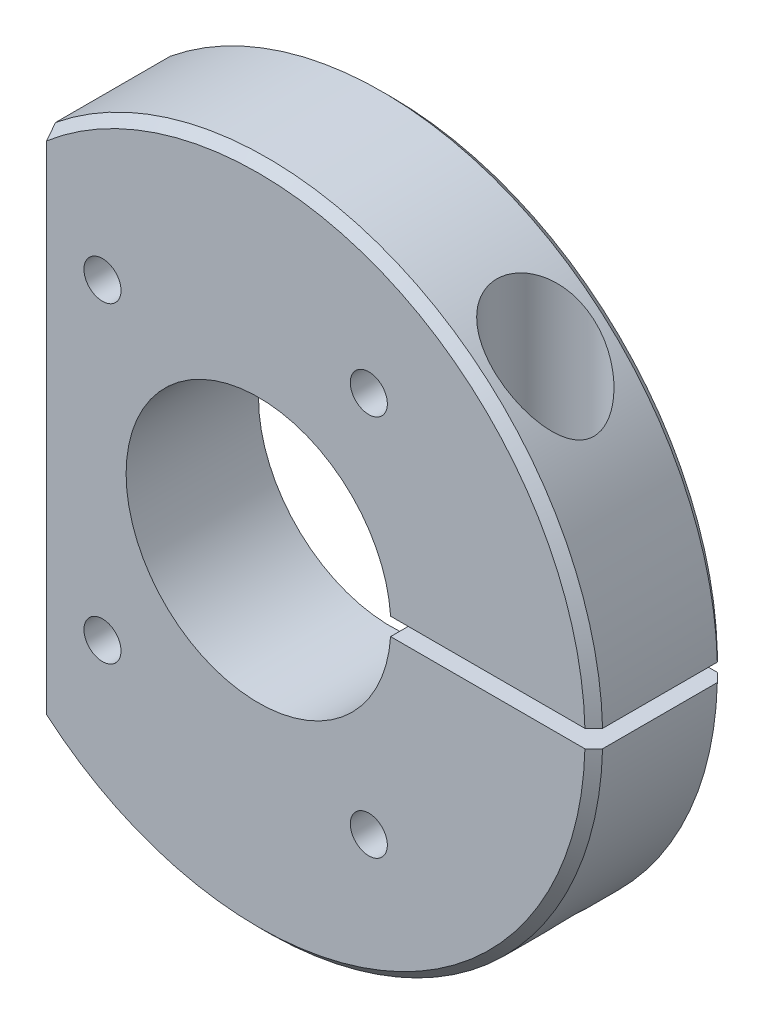
from build123d import *

# Parameters (mm, degrees)
EXTRUDE_1_DEPTH              = 15
CUT_EXTRUDE_1_DEPTH          = 56.794264938
SKETCH_3_W                   = 15
SKETCH_3_H                   = 15
HOLE_WIZARD_4_2_4_2_1_D      = 4.2
SKETCH_6_W                   = 2.5
SKETCH_6_H                   = 37
HOLE_WIZARD_M6_1_D           = 6.5
HOLE_WIZARD_M6_1_DEPTH       = 70.615180295
HOLE_WIZARD_M6_1_CBORE_D     = 11
HOLE_WIZARD_M6_1_CBORE_DEPTH = 24.615180295
CHAMFER_1_SIZE               = 1


with BuildPart() as part:
    # 草图1 → 凸台-拉伸1 (new body)
    with BuildSketch(Plane(origin=(0, 0, -7.5), x_dir=(-1, 0, 0), z_dir=(0, 0, -1))):
        with BuildLine():
            Line((24, -29.461839725), (24, 29.461839725))
            ThreePointArc((24, 29.461839725), (-38, 0), (24, -29.461839725))
        make_face()
    extrude(amount=-EXTRUDE_1_DEPTH)

    # 草图2 → 切除-拉伸1 (cut, through all)
    with BuildSketch(Plane.XY.offset(7.5)):
        with BuildLine():
            Line((37.986839826, 1), (14.966629547, 1))
            ThreePointArc((14.966629547, 1), (15, 0), (14.966629547, -1))
            Line((14.966629547, -1), (37.986839826, -1))
            ThreePointArc((37.986839826, -1), (38, 0), (37.986839826, 1))
        make_face()
    extrude(amount=-CUT_EXTRUDE_1_DEPTH, mode=Mode.SUBTRACT)

    # 草图3 → 切除-旋转1 (revolve, cut)
    with BuildSketch(Plane.XZ):
        with Locations((7.5, 0)):
            Rectangle(SKETCH_3_W, SKETCH_3_H)
    revolve(axis=Axis((0, 0, 7.5), (0, 0, -1)), mode=Mode.SUBTRACT)

    # Ø4.2 (4.2) 直径孔1 (through all)
    with Locations(Plane.XY.offset(7.5)):
        with Locations((-17.67766953, -17.67766953), (-17.67766953, 17.67766953), (12.5, 21.650635095), (12.5, -21.650635095)):
            Hole(HOLE_WIZARD_4_2_4_2_1_D / 2)

    # 草图6 → Ø5.0 (5) 直径孔1 (revolve, cut)
    with BuildSketch(Plane(origin=(25, -1, 0), x_dir=(0, 0, 1), z_dir=(1, 0, 0))):
        with Locations((1.25, 18.5)):
            Rectangle(SKETCH_6_W, SKETCH_6_H)
    revolve(axis=Axis((25, 5.35, 0), (0, -1, 0)), mode=Mode.SUBTRACT)

    # M6 六角头螺栓的柱形沉头孔1
    with Locations(Plane(origin=(0, 32.615180295, 0), x_dir=(1, 0, 0), z_dir=(0, 1, 0))):
        with Locations((25, 0)):
            CounterBoreHole(HOLE_WIZARD_M6_1_D / 2, HOLE_WIZARD_M6_1_CBORE_D / 2, HOLE_WIZARD_M6_1_CBORE_DEPTH, depth=HOLE_WIZARD_M6_1_DEPTH)

    # 倒角1
    chamfer_1_edges = [part.edges().sort_by_distance(p)[0] for p in [
        (15.856449862, -34.533650224, 7.5),
        (15.856449862, 34.533650224, -7.5),
        (15.856449862, 34.533650224, 7.5),
        (15.856449862, -34.533650224, -7.5),
    ]]
    chamfer(chamfer_1_edges, length=CHAMFER_1_SIZE)


solid = part.part
